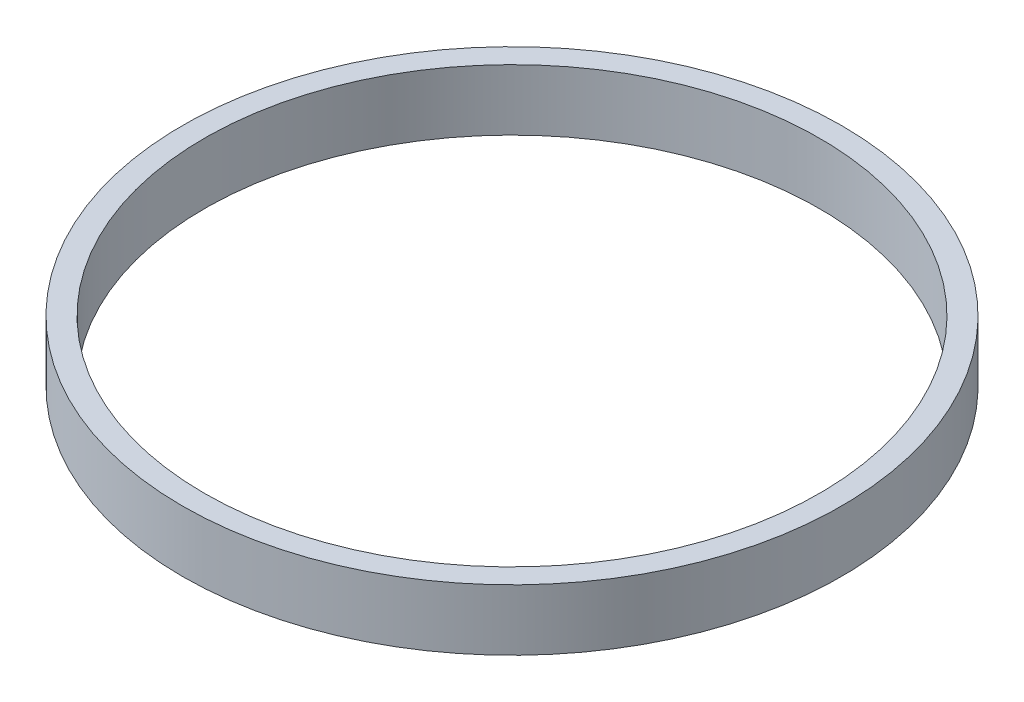
SolidWorks part; units mm, degrees
ref_plane "Front Plane" through (0, 0, 0) normal (0, 0, 1) x (1, 0, 0)
ref_plane "Top Plane" through (0, 0, 0) normal (0, 1, 0) x (1, 0, 0)
ref_plane "Right Plane" through (0, 0, 0) normal (1, 0, 0) x (0, 0, -1)
sketch "Sketch1" plane through (0, 0, 0) normal (0, 1, 0) x (1, 0, 0)
  circle A0 centre (0, 0) radius 13.5
  circle A1 centre (0, 0) radius 12.6
  dimension "D1" = 25.2
  dimension "D2" = 27
extrude "Boss-Extrude1" add sketch "Sketch1" along normal blind 2.5
